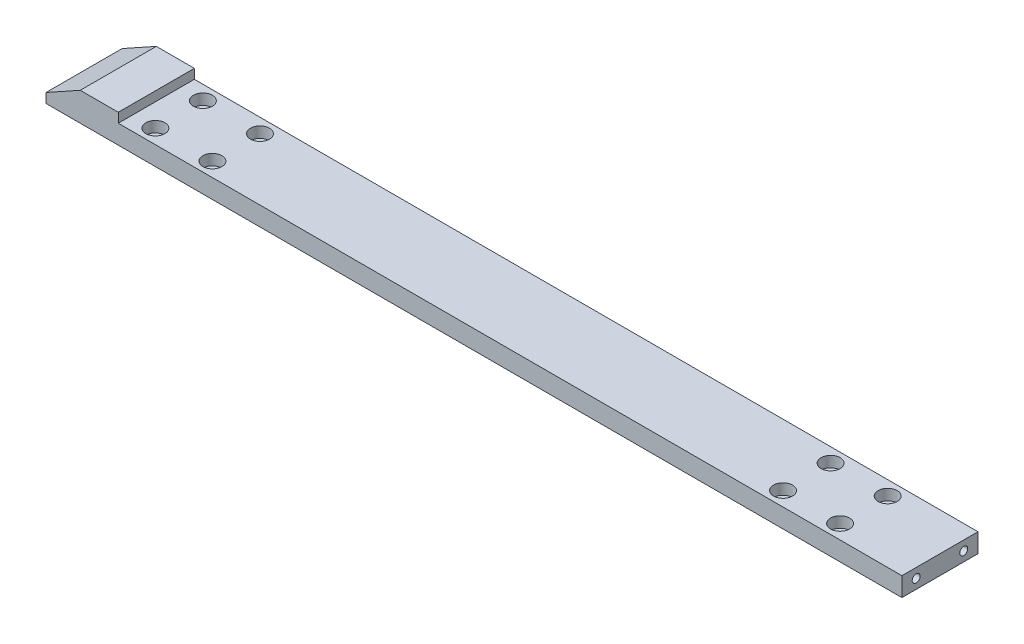
SolidWorks part; units mm, degrees
material "6061 合金"
ref_plane "前视基准面" through (0, 0, 0) normal (0, 0, 1) x (1, 0, 0)
ref_plane "上视基准面" through (0, 0, 0) normal (0, 1, 0) x (1, 0, 0)
ref_plane "右视基准面" through (0, 0, 0) normal (1, 0, 0) x (0, 0, -1)
sketch "草图1" plane through (0, 0, 0) normal (0, 0, 1) x (1, 0, 0)
  line L0 (0, 0) -> (450, 0)
  line L1 (450, 0) -> (450, 10)
  line L2 (450, 10) -> (38, 10)
  line L3 (38, 10) -> (38, 15)
  line L4 (38, 15) -> (18, 15)
  line L5 (18, 15) -> (0, 5)
  line L6 (0, 5) -> (0, 0)
  dimension "D1" = 450
  dimension "D2" = 10
  dimension "D3" = 38
  dimension "D4" = 5
  dimension "D5" = 5
  dimension "D6" = 20
extrude "凸台-拉伸1" add sketch "草图1" along normal mid plane 40
hole_wizard "打孔尺寸(%根据)内六角圆柱头螺钉的类型1" positions "草图6" profile "草图5" counterbore size "M5" standard "GB"
sketch "草图6" plane through (0, 10, 0) normal (0, 1, 0) x (1, 0, 0)
  line L0 (0, -20) -> (0, 20) construction
  line L1 (450, -20) -> (450, 20) construction
  line L2 (450, -20) -> (38, -20) construction
  point P0 (50, 12.5)
  point P2 (80, 12.5)
  point P4 (50, -12.5)
  point P6 (80, -12.5)
  point P8 (380, -12.5)
  point P10 (410, -12.5)
  point P12 (380, 12.5)
  point P14 (410, 12.5)
  dimension "D1" = 30
  dimension "D2" = 50
  dimension "D3" = 30
  dimension "D4" = 40
  dimension "D5" = 25
  dimension "D6" = 7.5
sketch "草图5" plane through (50, 10, -12.5) normal (1, 0, 0) x (0, 0, 1)
  line L0 (0, 0) -> (0, 15.6524)
  line L1 (0, 15.6524) -> (2.75, 14)
  line L2 (2.75, 14) -> (2.75, 5.7)
  line L3 (2.75, 5.7) -> (5, 5.7)
  line L4 (5, 5.7) -> (5, 0)
  line L5 (5, 0) -> (0, 0)
  line L10 (0, 15.6524) -> (-2.75, 14) construction
  line L11 (0, -6.35) -> (0, 107.95) construction
  dimension "孔直径" = 5.5
  dimension "孔深度" = 14
  dimension "柱形沉头孔直径" = 10
  dimension "柱形沉头孔深度" = 5.7
  dimension "导头角度" = 118
hole_wizard "M5 螺纹孔1" positions "草图10" profile "草图9" tap size "M5" standard "GB"
sketch "草图10" plane through (450, 0, 0) normal (1, 0, 0) x (0, 0, -1)
  line L0 (-20, 0) -> (-20, 10) construction
  line L1 (-20, 0) -> (20, 0) construction
  point P0 (-12.5, 5)
  point P2 (12.5, 5)
  dimension "D1" = 25
  dimension "D2" = 7.5
  dimension "D3" = 5
sketch "草图9" plane through (450, 5, 12.5) normal (0, 1, 0) x (0, 0, -1)
  line L0 (0, 0) -> (0, 15.2618)
  line L1 (0, 15.2618) -> (2.1, 14)
  line L2 (2.1, 14) -> (2.1, 0)
  line L5 (2.1, 0) -> (0, 0)
  line L10 (0, 15.2618) -> (-2.1, 14) construction
  line L11 (0, -6.35) -> (0, 107.95) construction
  dimension "螺纹孔钻头直径" = 4.2
  dimension "螺纹孔钻头深度" = 14
  dimension "导头角度" = 118
cosmetic thread "孔螺蚊线1"
cosmetic thread "孔螺蚊线2"
